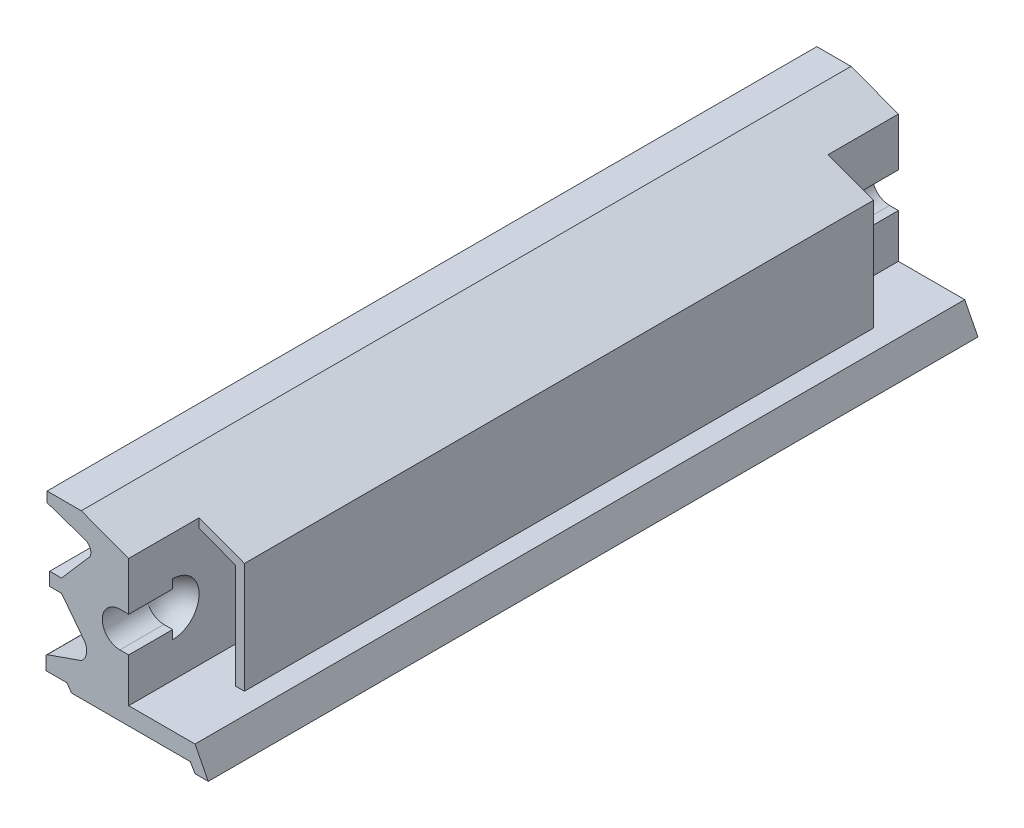
SolidWorks part; units mm, degrees
ref_plane "前视基准面" through (0, 0, 0) normal (0, 0, 1) x (1, 0, 0)
ref_plane "上视基准面" through (0, 0, 0) normal (0, 1, 0) x (1, 0, 0)
ref_plane "右视基准面" through (0, 0, 0) normal (1, 0, 0) x (0, 0, -1)
sketch "草图1" plane through (0, 0, 0) normal (0, 0, 1) x (1, 0, 0)
  line L0 (0, -144.4959) -> (-130, -144.4959)
  line L1 (-130, -144.4959) -> (-140.2996, -129.4959)
  line L14 (0, 185.5041) -> (0, 75.5041)
  line L18 (-187.997, -129.4959) -> (-187.997, -99.4959)
  line L23 (-140.2996, -129.4959) -> (-187.997, -129.4959)
  line L30 (-152.7072, 40.5078) -> (-179.7072, 40.5078)
  line L31 (-179.7072, 40.5078) -> (-179.7072, 70.5078)
  line L33 (-102.0084, -25.2038) -> (-152.7072, 40.5078)
  line L35 (-179.7072, 70.5078) -> (-152.7072, 70.5078)
  line L36 (-185.4969, 225.5078) -> (-107.7769, 225.5078)
  line L39 (-185.4969, 202.5078) -> (-185.4969, 225.5078)
  line L40 (-107.7769, 225.5078) -> (0, 185.5041)
  line L41 (0, -4.4959) -> (0, -104.4959)
  line L44 (140, -144.4959) -> (0, -144.4959)
  line L56 (140, -144.4959) -> (150.7723, -162.9995)
  line L57 (150.7723, -162.9995) -> (180.9476, -162.9995)
  line L58 (180.9476, -162.9995) -> (150.7723, -104.4959)
  line L59 (0, -104.4959) -> (150.7723, -104.4959)
  line L60 (-185.4969, -96.731) -> (-107.72, -69.4922)
  line L62 (-99.7072, 172.9825) -> (-185.4969, 202.5078)
  line L63 (0, 75.5041) -> (0, -4.4959)
  line L64 (-92.3167, 140.1086) -> (-152.7072, 70.5078)
  arc A4 (-107.72, -69.4922) -> (-102.0084, -25.2038) centre (-127.0084, -44.4922) ccw
  spline S0 degree 2 poles (-187.997, -99.4959) (-187.2639, -97.6837) (-185.4969, -96.731) knots 0 0 0 1 1 1
  spline S1 degree 3 poles (-99.7072, 172.9825) (-86.1247, 169.5466) (-80.8546, 148.9633) (-92.3167, 140.1086) knots 0 0 0 0 1 1 1 1
extrude "凸台-拉伸1" add sketch "草图1" against normal blind 1750
sketch "草图2" plane through (0, 0, 0) normal (0, 0, 1) x (1, 0, 0)
  line L0 (0, 75.5041) -> (0, -4.4959)
  line L1 (0, 185.5041) -> (0, -104.4959) construction
  line L2 (0, -4.4959) -> (-20, -4.4959)
  line L3 (-20, 75.5041) -> (0, 75.5041)
  arc A0 (-20, -4.4959) -> (-20, 75.5041) centre (-20, 35.5041) cw
extrude "切除-拉伸2" cut sketch "草图2" against normal blind 100
sketch3d "3D草图1"
  point P0 (-64.3757, 34.3747, -100)
ref_plane "基准面1" through (0, 0, -100) normal (0, 0, 1) x (1, 0, 0)
sketch3d "3D草图2"
  point P0 (0, 133.2456, -230.8006)
ref_plane "基准面2" through (0, 0, 0) normal (1, 0, 0) x (0, 0, -1)
sketch "草图4" plane through (0, 0, 0) normal (1, 0, 0) x (0, 0, -1)
  line L1 (100, 95.5041) -> (100, -24.4959)
  arc A1 (100, 95.5041) -> (100, -24.4959) centre (100, 35.5041) cw
revolve "切除-旋转1" cut sketch "草图4" angle 90 about L1
ref_plane "基准面3" through (0, 0, -875) normal (0, 0, 1) x (1, 0, 0)
mirror "镜向1" about plane through (0, 0, -875) normal (0, 0, 1) of "切除-拉伸2", "切除-旋转1"
ref_plane "基准面4" through (0, 0, -160) normal (0, 0, 1) x (1, 0, 0)
sketch "草图6" plane through (0, 0, -160) normal (0, 0, 1) x (1, 0, 0)
  line L0 (0, 185.5041) -> (63.2072, 162.0433)
  line L1 (63.2072, 162.0433) -> (103.143, 147.2203)
  line L2 (103.143, 147.2203) -> (103.143, -104.4959)
  line L3 (0, -104.4959) -> (150.7723, -104.4959) construction
  line L4 (103.143, -104.4959) -> (83.1751, -104.4959)
  line L5 (83.1751, -104.4959) -> (83.1751, 133.726)
  line L6 (83.1751, 133.726) -> (0, 164.5983)
  line L7 (0, 185.5041) -> (0, 75.5041) construction
  line L8 (0, 164.5983) -> (0, 185.5041)
  point P12 (0, 0)
extrude "凸台-拉伸2" add sketch "草图6" against normal blind 1430
